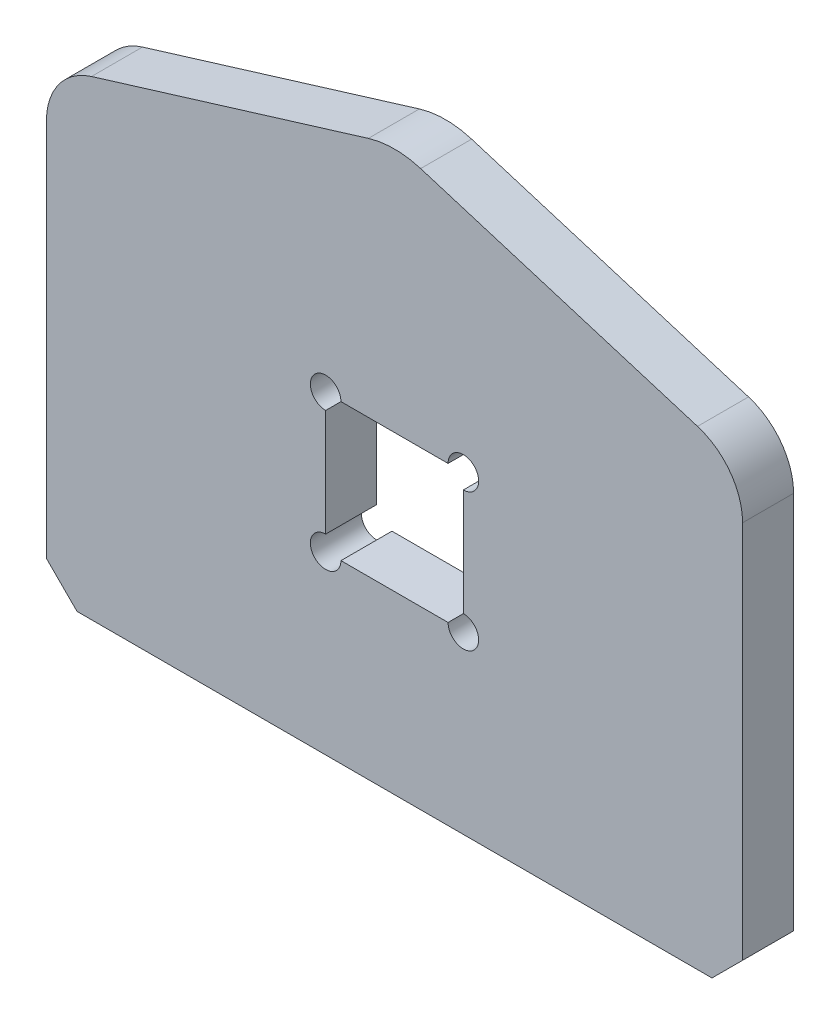
SolidWorks part; units mm, degrees
ref_plane "Front Plane" through (0, 0, 0) normal (0, 0, 1) x (1, 0, 0)
ref_plane "Top Plane" through (0, 0, 0) normal (0, 1, 0) x (1, 0, 0)
ref_plane "Right Plane" through (0, 0, 0) normal (1, 0, 0) x (0, 0, -1)
sketch "Sketch1" plane through (0, 0, 0) normal (0, 0, 1) x (1, 0, 0)
  line L0 (-124.5, 0) -> (124.5, 0)
  line L1 (136.5, 12) -> (136.5, 160.6)
  line L2 (0, 0) -> (0, 230.7339) construction
  line L3 (10.2522, 217.7648) -> (118.823, 184.5034)
  line L4 (124.5, 0) -> (136.5, 12)
  line L5 (-21, 123) -> (21, 123)
  line L6 (27, 117) -> (27, 75)
  line L7 (21, 69) -> (-21, 69)
  line L8 (-27, 117) -> (-27, 75)
  line L9 (-136.5, 12) -> (-136.5, 160.6)
  line L10 (-10.2522, 217.7648) -> (-118.823, 184.5034)
  line L11 (-124.5, 0) -> (-136.5, 12)
  arc A0 (10.2522, 217.7648) -> (-10.2522, 217.7648) centre (0, 184.3) ccw
  arc A1 (136.5, 160.6) -> (118.823, 184.5034) centre (111.5, 160.6) ccw
  arc A2 (27, 117) -> (21, 123) centre (27, 123) ccw
  arc A3 (21, 69) -> (27, 75) centre (27, 69) ccw
  arc A4 (-21, 69) -> (-27, 75) centre (-27, 69) cw
  arc A5 (-27, 117) -> (-21, 123) centre (-27, 123) cw
  arc A6 (-136.5, 160.6) -> (-118.823, 184.5034) centre (-111.5, 160.6) cw
  point P1 (136.5, 0)
  point P6 (124.5, 12)
  point P16 (0, 123)
  point P26 (0, 69)
  point P32 (-124.5, 12)
  point P33 (-136.5, 0)
  dimension "D2" = 70
  dimension "D5" = 50
  dimension "D10" = 12
  dimension "D11" = 12
  dimension "D1" = 184.3
  dimension "D3" = 273
  dimension "D4" = 160.6
  dimension "D6" = 69
  dimension "D7" = 54
  dimension "D9" = 27
extrude "Boss-Extrude1" add sketch "Sketch1" along normal blind 20
